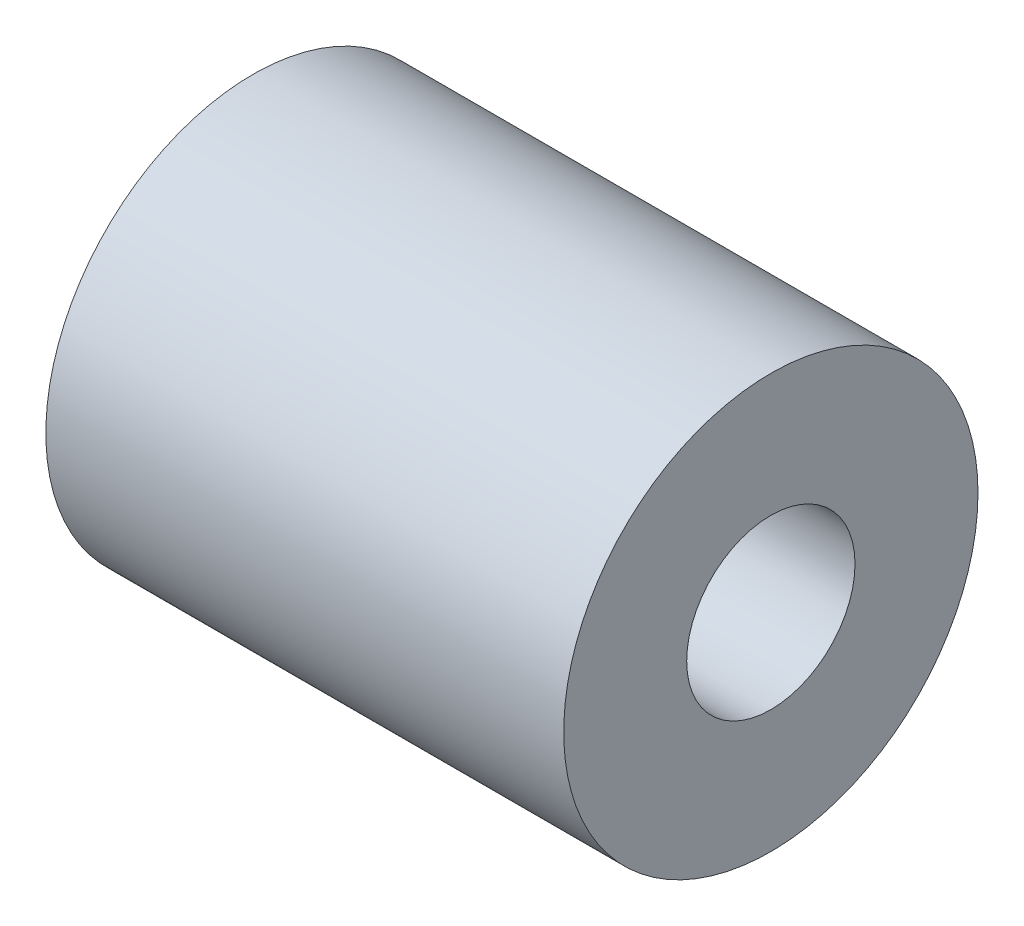
from build123d import *

# Parameters (mm, degrees)
SKETCH_1_R      = 8
SKETCH_1_R_2    = 3.25
EXTRUDE_1_DEPTH = 20


with BuildPart() as part:
    # 草图1 → 凸台-拉伸1 (new body)
    with BuildSketch(Plane(origin=(0, 0, 0), x_dir=(0, 0, -1), z_dir=(1, 0, 0))):
        Circle(SKETCH_1_R)
        Circle(SKETCH_1_R_2, mode=Mode.SUBTRACT)
    extrude(amount=EXTRUDE_1_DEPTH)


solid = part.part
